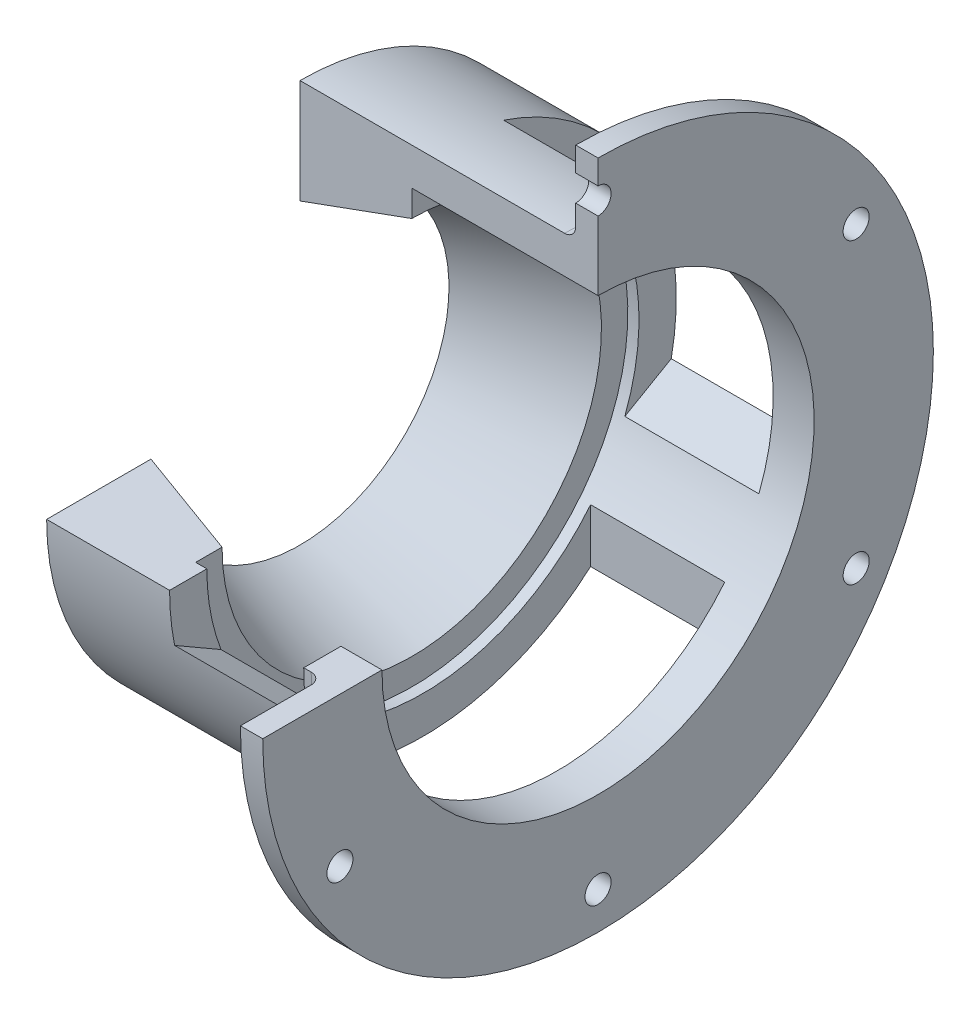
from build123d import *

# Parameters (mm, degrees)
SKETCH2_R          = 3.5
CUT_EXTRUDE1_DEPTH = 10
FILLET1_R          = 3
SKETCH3_W          = 36
SKETCH3_H          = 90
CUT_EXTRUDE2_DEPTH = 151.332963784
CIRPATTERN1_COUNT  = 3
SKETCH4_W          = 114.578796514
SKETCH4_H          = 147.158368746
CUT_EXTRUDE3_DEPTH = 151.332963784


with BuildPart() as part:
    # Sketch1 → Revolve1 (revolve)
    with BuildSketch(Plane.XY, mode=Mode.PRIVATE) as revolve1_sk:
        Polygon((0, 40), (0, 68), (74, 68), (74, 90), (80, 90), (80, 58), (30, 58), (30, 50.919107028), align=None)
    revolve(revolve1_sk.sketch.rotate(Axis((0, 0, 0), (1, 0, 0)), 90), axis=Axis((0, 0, 0), (1, 0, 0)))

    # Sketch2 → Cut-Extrude1 (cut)
    with BuildSketch(Plane(origin=(80, 0, 0), x_dir=(0, 0, -1), z_dir=(1, 0, 0))):
        with Locations((0, 80)):
            Circle(SKETCH2_R)
        with Locations((69.282032303, 40)):
            Circle(SKETCH2_R)
        with Locations((69.282032303, -40)):
            Circle(SKETCH2_R)
        with Locations((0, -80)):
            Circle(SKETCH2_R)
        with Locations((-69.282032303, -40)):
            Circle(SKETCH2_R)
        with Locations((-69.282032303, 40)):
            Circle(SKETCH2_R)
    extrude(amount=-CUT_EXTRUDE1_DEPTH, mode=Mode.SUBTRACT)

    # Fillet1
    fillet1_edges = [part.edges().sort_by_distance(p)[0] for p in [
        (74, 0, -68),
    ]]
    fillet(fillet1_edges, radius=FILLET1_R)

    # Sketch3 → Cut-Extrude2 (cut, through all)
    with BuildSketch(Plane(origin=(0, 0, 0), x_dir=(1, 0, 0), z_dir=(0, 1, 0))):
        with Locations((51, 0)):
            Rectangle(SKETCH3_W, SKETCH3_H)
    cut_extrude2 = extrude(amount=-CUT_EXTRUDE2_DEPTH, mode=Mode.SUBTRACT)

    # CirPattern1: Cut-Extrude2 ×3 about axis
    cirpattern1_axis = Axis((0, 0, 0), (1, 0, 0))
    for i in range(1, CIRPATTERN1_COUNT):
        add(cut_extrude2.rotate(cirpattern1_axis, i * 360 / CIRPATTERN1_COUNT), mode=Mode.SUBTRACT)

    # Sketch4 → Cut-Extrude3 (cut, through all)
    with BuildSketch(Plane.ZY):
        with Locations((57.289398257, 73.579184373)):
            Rectangle(SKETCH4_W, SKETCH4_H)
    extrude(amount=-CUT_EXTRUDE3_DEPTH, mode=Mode.SUBTRACT)


solid = part.part
